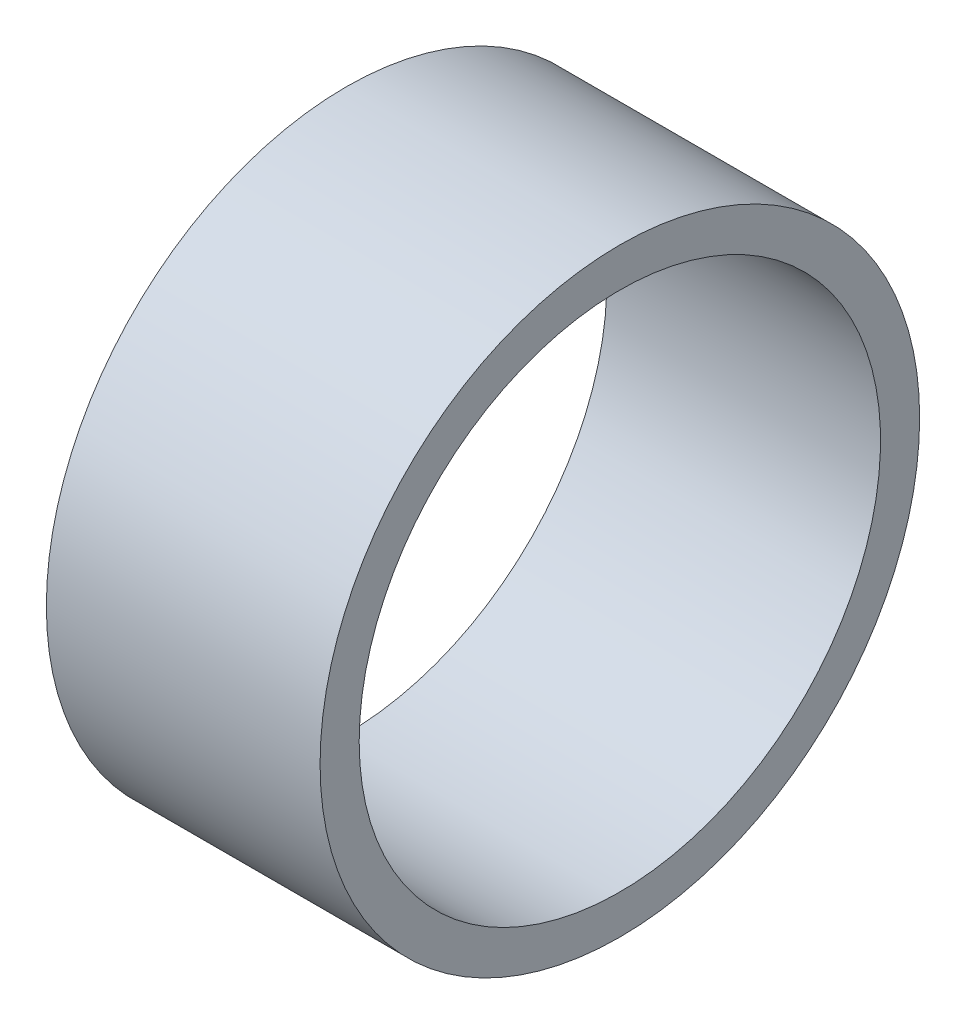
SolidWorks part; units mm, degrees
ref_plane "前视基准面" through (0, 0, 0) normal (0, 0, 1) x (1, 0, 0)
ref_plane "上视基准面" through (0, 0, 0) normal (0, 1, 0) x (1, 0, 0)
ref_plane "右视基准面" through (0, 0, 0) normal (1, 0, 0) x (0, 0, -1)
sketch "草图1" plane through (0, 0, 0) normal (1, 0, 0) x (0, 0, -1)
  circle A0 centre (0, 0) radius 20
  circle A1 centre (0, 0) radius 23
extrude "凸台-拉伸1" add sketch "草图1" along normal blind 21
